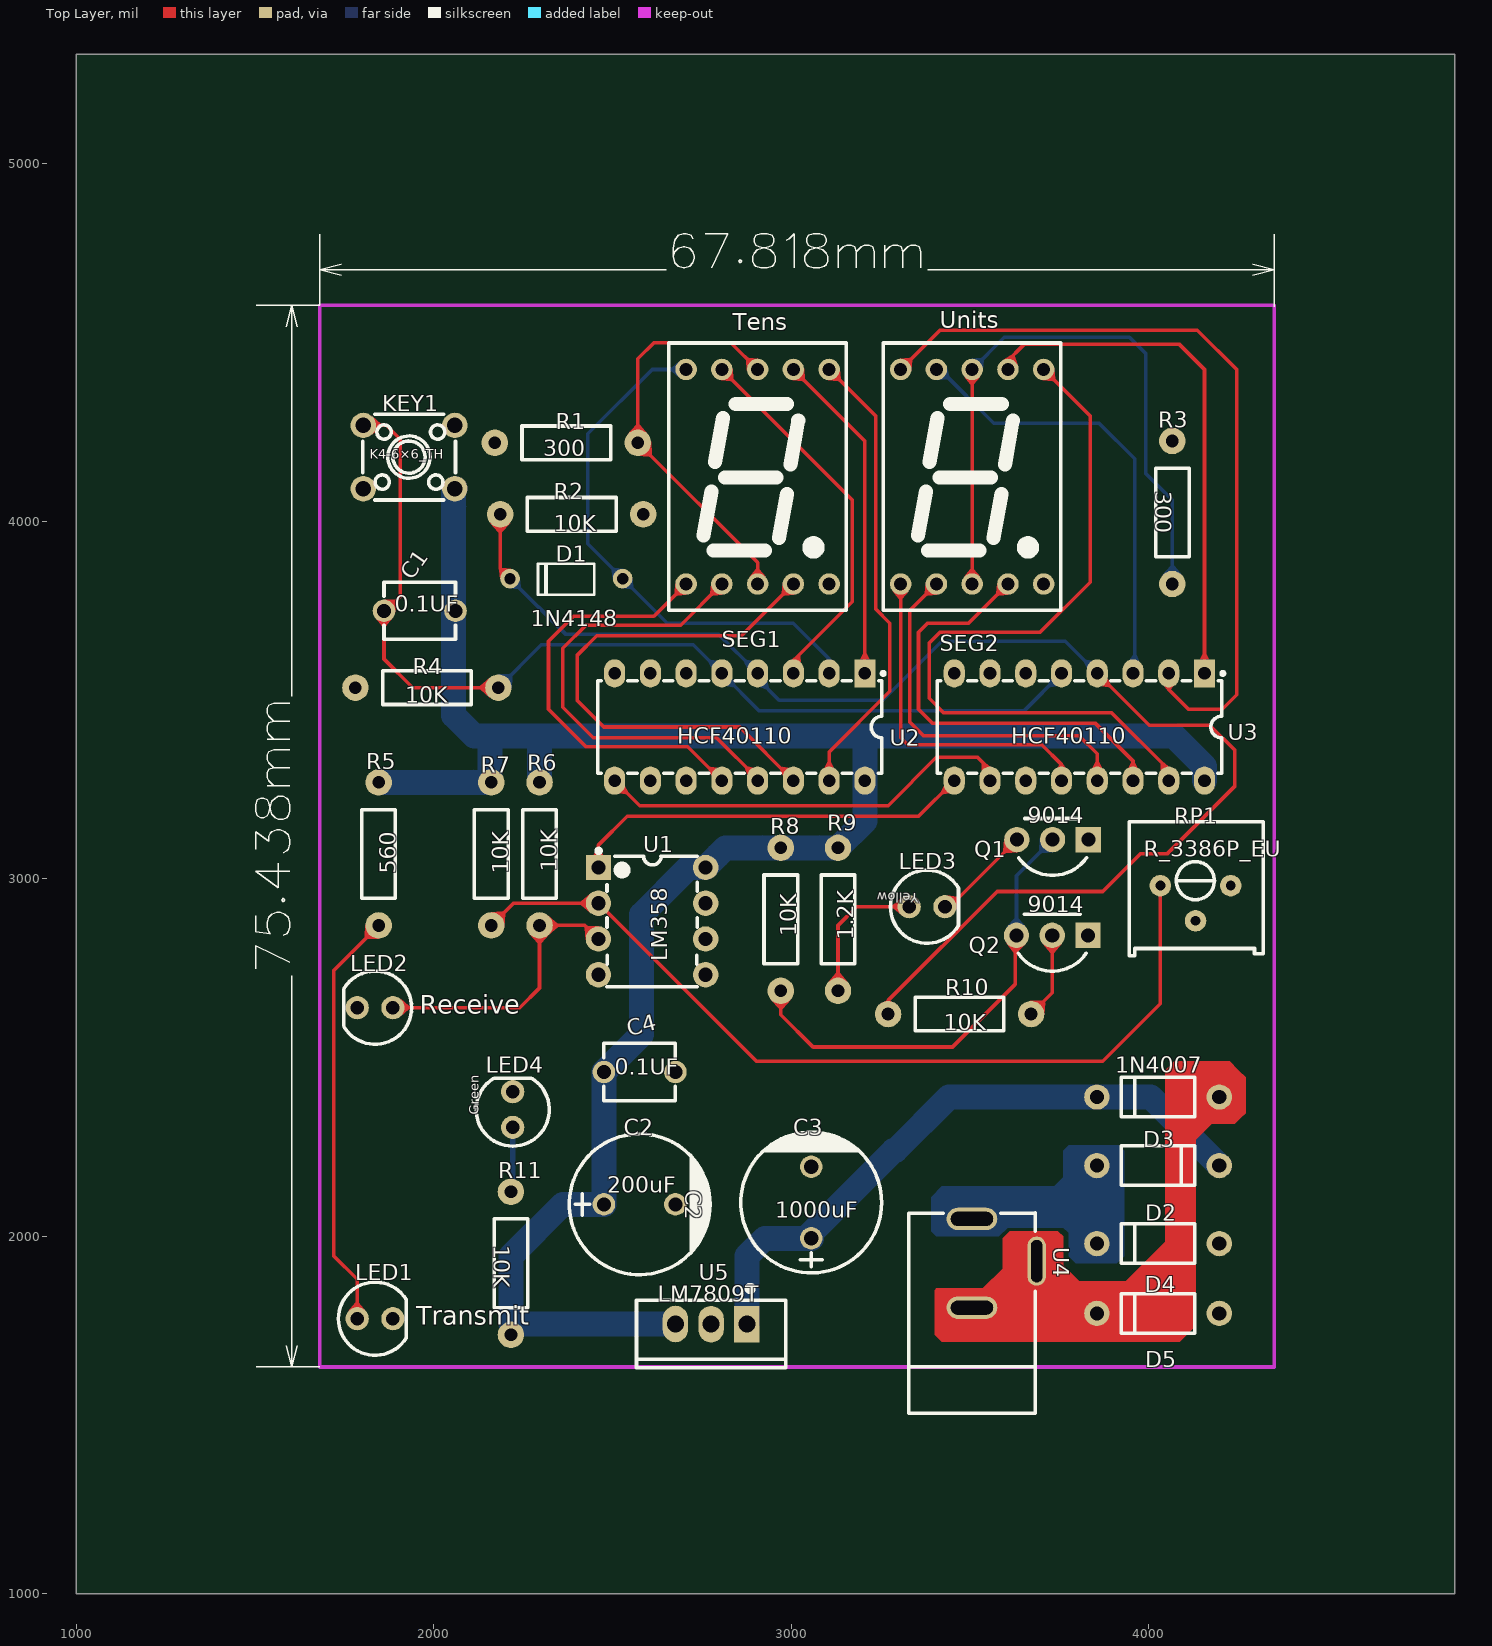
[diagram p0: Top Layer view]
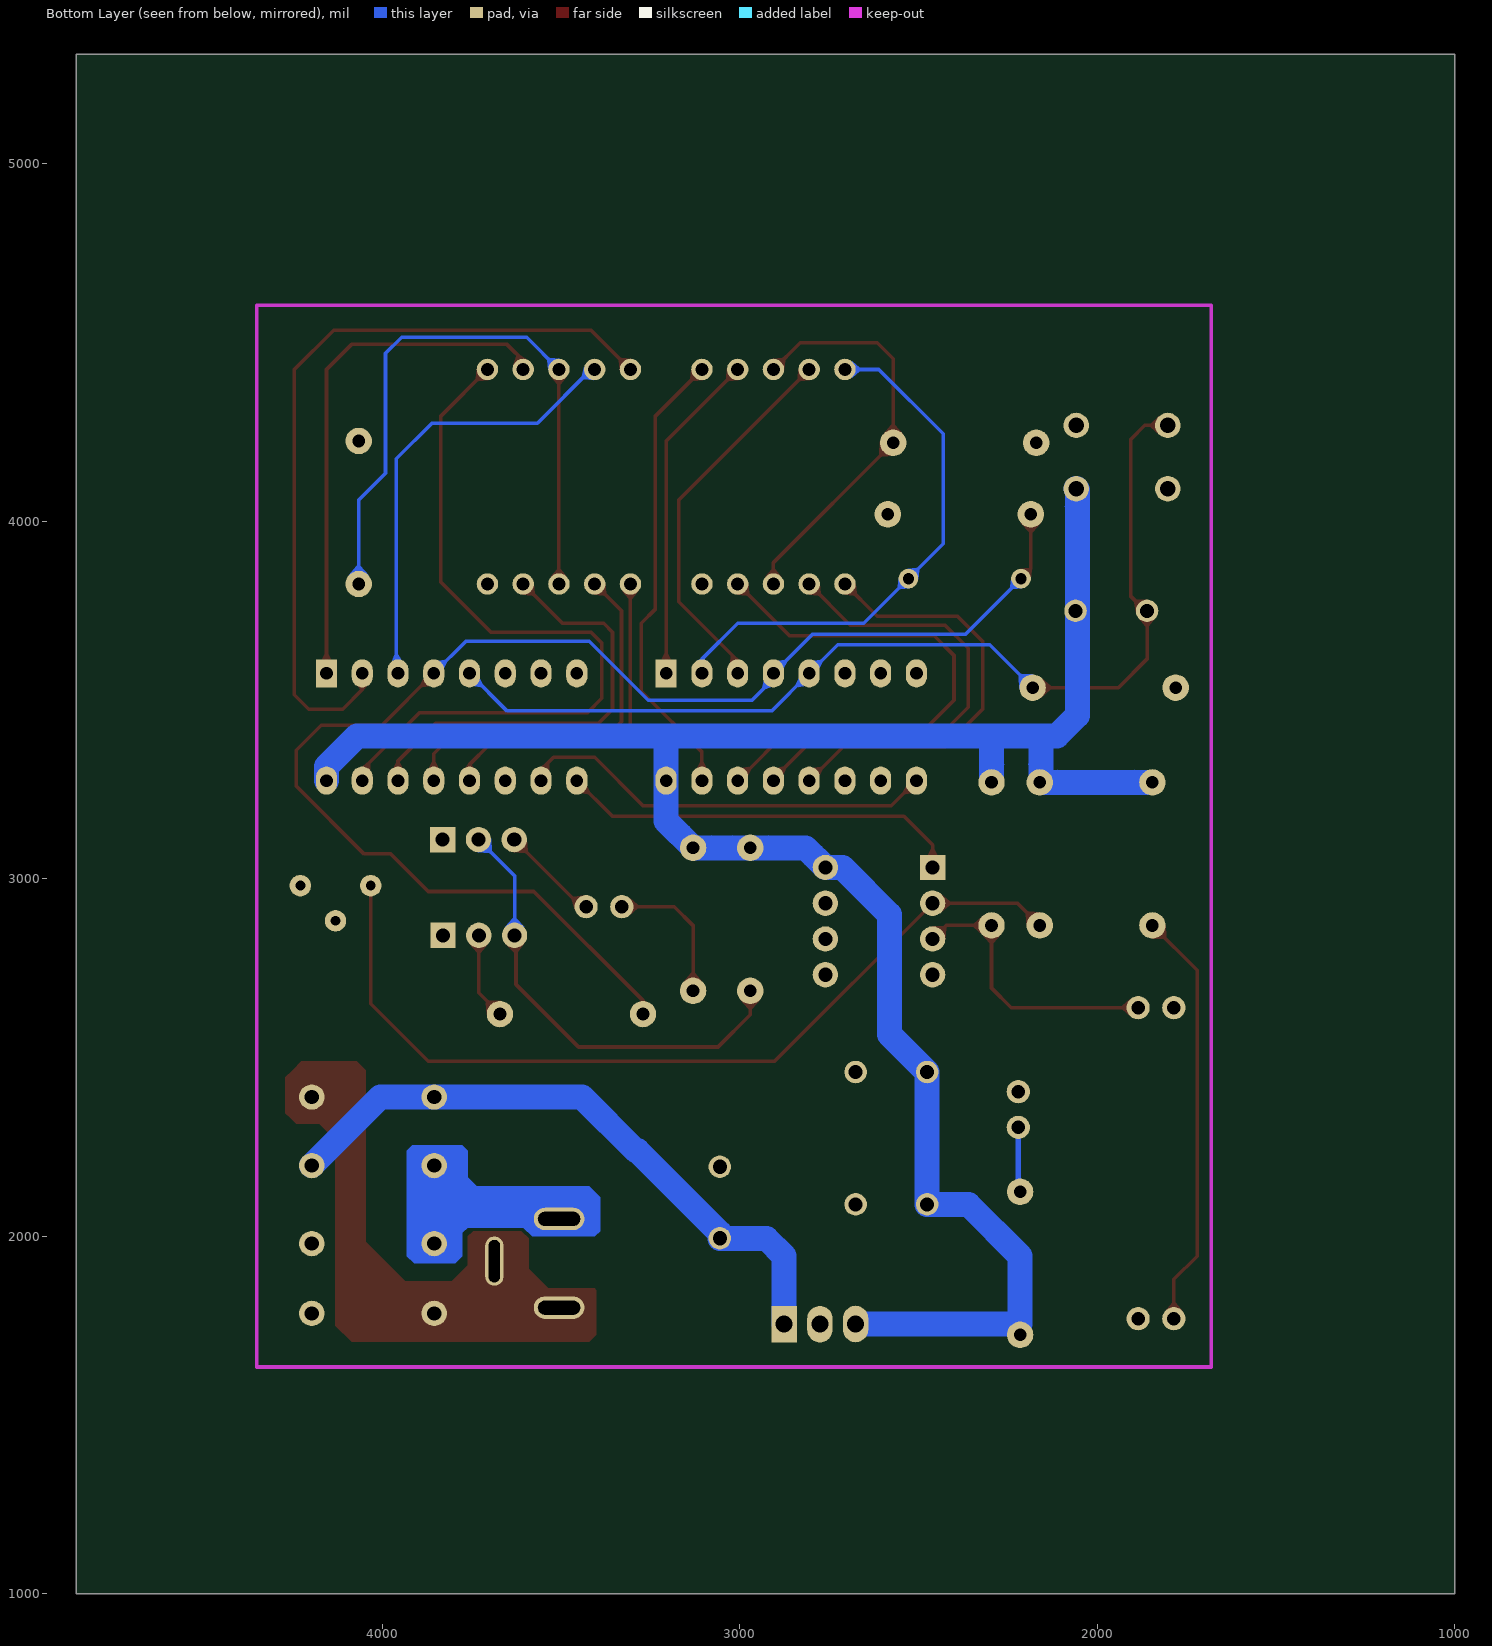
[diagram p1: Bottom Layer view, seen from below]
# Altium PCB MISC82671.pcbdoc
Units mil, origin at the board's own origin, x right, y up, seen from the top; angles counter-clockwise.
Board outline 3855.81 x 4306 mil, 2 copper layers (Top Layer, Bottom Layer); 37 components, 40 nets, 127 pads, 0 vias.

## Layer stack, top to bottom (the 12.6 mil dielectric is the usual default, probably not edited)
Top Solder: solder mask 0.4, Solder Resist, Dk 3.5
Top Layer: signal copper 1.4
Dielectric1: dielectric 12.6, FR-4, Dk 4.8
Bottom Layer: signal copper 1.4
Bottom Solder: solder mask 0.4, Solder Resist, Dk 3.5

## Board outline
4855.81,1000 1000,1000 1000,5306 4855.81,5306

## Design rules (kind name [scope] priority, off if disabled: settings)
Clearance [All] p1: gap=10
PolygonConnect [All] p1: connectstyle=Relief reliefconductorwidth=10 reliefentries=4 polygonreliefangle="90 Angle" airgapwidth=10
RoutingVias [All] p1: holewidth=28 width=50 viastyle="Through Hole" minholewidth=28 minwidth=50 maxholewidth=28 maxwidth=50
SolderMaskExpansion [All] p1: expansion=4
Width [All] p1: maxlimit=10 minlimit=10 preferedwidth=10
30 further rules are at their usual default settings.

## Components (designator, comment, footprint, x,y, rotation, side; value= is the part's Value field where it differs from the comment)
C1 "0.1UF" CAP-TH_L5.0-W4.0-P5.00-D1.0 1960.81,3749.3 r0 top
C2 "200uF" CAP-TH_BD10.0-P5.00-D1.0-FD 2575.81,2089.3 r0 top
C3 "1000uF" CAP-TH_BD10.0-P5.00-D1.0-FD 3055.81,2094.3 r90 top
C4 "0.1UF" CAP-TH_L5.0-W4.0-P5.00-D1.0 2575.81,2459.3 r180 top
D1 "1N4148" DO-35_BD2.2-L4.0-D0.50_1N4148 2370.81,3839.3 r180 top
D2 "1N4007" DO-41_BD2.4-L4.7-P8.70-D0.9-FD 4025.81,2197.52 r0 top
D3 "1N4007" DO-41_BD2.4-L4.7-P8.70-D0.9-FD 4025.81,2389.3 r180 top
D4 "1N4007" DO-41_BD2.4-L4.7-P8.70-D0.9-FD 4025.81,1979.3 r180 top
D5 "1N4007" DO-41_BD2.4-L4.7-P8.70-D0.9-FD 4025.81,1784.3 r180 top
KEY1 "K4-6×6_TH" KEY-TH_4P-L6.0-W6.0-P4.50-LS6.5 1930.81,4179.3 r180 top
LED1 "LED-TH-5mm_R" LED-TH_BD5.0_RED 1835.81,1769.3 r90 top
LED2 "LED-TH-5mm_R" LED-TH_BD5.0_RED 1835.81,2639.3 r270 top
LED3 "Yellow" LED-TH_BD5.0_RED 3379.83,2921.68 r90 top
LED4 "Green" LED-TH_BD5.0_RED 2220.81,2354.3 r180 top
Q1 "9014" TO-92-3_L4.9-W3.7-P2.54-L 3730.81,3109.3 r180 top
Q2 "9014" TO-92-3_L4.9-W3.7-P2.54-L 3729.83,2841.68 r180 top
R1 "300" R_AXIAL-0.4 2370.81,4219.3 r0 top
R2 "10K" R_AXIAL-0.4 2385.81,4019.3 r0 top
R3 "300" R_AXIAL-0.4 4065.81,4024.3 r270 top
R4 "10K" R_AXIAL-0.4 1980.81,3534.3 r0 top
R5 "560" R_AXIAL-0.4 1845.81,3069.3 r90 top
R6 "10K" R_AXIAL-0.4 2295.81,3069.3 r90 top
R7 "10K" R_AXIAL-0.4 2160.81,3069.3 r90 top
R8 "10K" R_AXIAL-0.4 2970.61,2886.38 r90 top
R9 "1.2K" R_AXIAL-0.4 3130.61,2886.38 r90 top
R10 "10K" R_AXIAL-0.4 3470.61,2621.38 r180 top
R11 "10K" R_AXIAL-0.4 2215.81,1924.3 r270 top
RP1 "R_3386P_EU" RES-ADJ-TH_3386P 4130.63,2931.41 r180 top
SEG1 "SEG-TH_0.56×1_Cathode" LED-SEG-TH_10P-L12.6-W19.0-P2.54-S15.24-BL 2905.81,4124.3 r0 top
SEG2 "SEG-TH_0.56×1_Cathode" LED-SEG-TH_10P-L12.6-W19.0-P2.54-S15.24-BL 3505.81,4124.3 r0 top
U1 "LM358" DIP-8_L8.8-W6.4-P2.54-LS7.6-BL 2610.61,2881.38 r270 top
U2 "HCF40110" DIP-16_16P-L20.2-W6.6-P2.54-LS7.6-BL 2855.81,3424.3 r180 top
U3 "HCF40110" DIP-16_16P-L20.2-W6.6-P2.54-LS7.6-BL 3805.81,3424.3 r180 top
U4 "HX DC005-2.5" DC-IN-TH_HX-DC005-2.5 3595.81,1924.3 r90 top
U5 "LM7809T" TO-220-3_L10.0-W4.5-P2.54-L 2775.81,1754.3 r180 top
? "" ? 1591.4,3119.3 r0 top
? "" ? 3015.81,4701.65 r0 top

## Footprints (in the part's own frame and the unit in brackets; to place one, negate y for a bottom-side part, rotate by r counter-clockwise, add the part's x,y. Pads: shape width x height; smd on the part's side, far side on the other; paste and mask are expansions set on the pad)
CAP-TH_BD10.0-P5.00-D1.0-FD [mm]
  round 1.6 hole 1 paste+0 mask+0.051: 1(-2.54,0) 2(2.54,0)
  silkscreen extent -5,-5 5.08,5
CAP-TH_L5.0-W4.0-P5.00-D1.0 [mm]
  round 1.6 hole 1 paste+0 mask+0.051: 1(-2.54,0) 2(2.54,0)
  silkscreen extent -2.54,-2.03 2.54,2.03
DC-IN-TH_HX-DC005-2.5 [mm]
  oval 3.5x1.3 hole 0.8 slot 3 at 0 deg paste+0 mask+0.05: 2(0.155,-2.3)
  oval 1.6x3.6 hole 1 slot 3 at 90 deg paste+0 mask+0.05: 3(-3.15,2.3) 4(3.15,2.3)
  silkscreen extent -10.65,-2.2 3.57,6.8
DIP-8_L8.8-W6.4-P2.54-LS7.6-BL [mm]
  rect 1.8x1.8 hole 1 paste+0 mask+0.051: 1(-3.81,-3.81)
  round 1.8 hole 1 paste+0 mask+0.051: 2(-1.27,-3.81) 3(1.27,-3.81) 4(3.81,-3.81) 5(3.81,3.81) 6(1.27,3.81) 7(-1.27,3.81) 8(-3.81,3.81)
  silkscreen extent -5.14,-3.95 4.66,3.2
DIP-16_16P-L20.2-W6.6-P2.54-LS7.6-BL [mm]
  rect 1.5x2 hole 0.9 paste+0 mask+0.051: 1(-8.89,-3.81)
  oval 1.5x2 hole 0.9 paste+0 mask+0.051: 2(-6.35,-3.81) 3(-3.81,-3.81) 4(-1.27,-3.81) 5(1.27,-3.81) 6(3.81,-3.81) 7(6.35,-3.81) 8(8.89,-3.81) 9(8.89,3.81) 10(6.35,3.81) 11(3.81,3.81) 12(1.27,3.81) 13(-1.27,3.81) 14(-3.81,3.81) 15(-6.35,3.81) 16(-8.89,3.81)
  silkscreen extent -10.31,-3.93 10.1,3.3
DO-35_BD2.2-L4.0-D0.50_1N4148 [mm]
  round 1.4 hole 0.8 paste+0 mask+0.05: 1(-4,0) 2(4,0)
  silkscreen extent -1.98,-1.06 2.02,1.14
DO-41_BD2.4-L4.7-P8.70-D0.9-FD [mm]
  round 1.8 hole 1 paste+0 mask+0.051: 1(-4.35,0) 2(4.35,0)
  silkscreen extent -2.6,-1.4 2.6,1.4
KEY-TH_4P-L6.0-W6.0-P4.50-LS6.5 [mm]
  round 1.8 hole 1.1 paste+0 mask+0.051: 1(-3.251,-2.25) 2(3.251,-2.25) 3(3.251,2.25) 4(-3.251,2.25)
  silkscreen extent -3.3,-3.05 3.3,3.05
LED-SEG-TH_10P-L12.6-W19.0-P2.54-S15.24-BL [mil]
  round 60 hole 36 paste+0 mask+2: 1(-200,-300) 2(-100,-300) 3(0,-300) 4(100,-300) 5(200,-300) 6(200,300) 7(100,300) 8(0,300) 9(-100,300) 10(-200,300)
  silkscreen extent -248,-374 248,374
LED-TH_BD5.0_RED [mil]
  round 65 hole 38 paste+0 mask+2: 1(0,50) 2(0,-50)
  silkscreen extent -102,-88 102,102
R_AXIAL-0.4 [mil]
  round 74 hole 35.4 paste+0 mask+2: 1(-200,0) 2(200,0)
  silkscreen extent -124,-47 124,47
RES-ADJ-TH_3386P [mil]
  round 60 hole 27.56 paste+0 mask+2: 1(98.43,-49.21) 2(0.01,49.22) 3(-98.42,-49.21)
  silkscreen extent -190,-228 185,147
TO-92-3_L4.9-W3.7-P2.54-L [mm]
  rect 1.8x1.8 hole 1 paste+0 mask+0.051: 1(-2.54,0)
  round 1.8 hole 1 paste+0 mask+0.051: 2(0,0) 3(2.54,0)
  silkscreen extent -2.41,-1.5 2.41,2.54
TO-220-3_L10.0-W4.5-P2.54-L [mm]
  rect 1.8x2.6 hole 1.2 paste+0 mask+0.051: 1(-2.54,0.005)
  oval 1.8x2.6 hole 1.2 paste+0 mask+0.051: 2(0,0.005) 3(2.54,-0.005)
  silkscreen extent -5.3,-2.73 5.3,3.09
? [mil]
  silkscreen extent -89,-1485 89,1485

## Nets (pads, with @x,y where several pads share a name; then routed paths per layer and width w, separated by ;. In a path a pad name is that pad's centre, name@x,y a point inside that pad or via, vN(x,y) a via of type N, cw(c..) or ccw(c..) an arc to the next point about the centre after c; other vN are vias at no path point)
+9V: C1.2 C2.1 C4.2 KEY1.4 R5.2 R6.2 R7.2 R8.2 R9.2 R11.2 U1.8 U2.16 U3.16 U5.3 | length 6205.2
  Bottom Layer w70: R5.2 R7.2 2157.67,3272.44 2157.67,3399.3 ; KEY1.4 2055.81,4087.7 2055.81,3456.7 2113.21,3399.3 4070.81,3399.3 4155.81,3314.3 U3.16 ; R6.2 2295.81,3399.3 ; U5.3 2215.81,1754.49 2215.81,1944.3 2360.81,2089.3 C2.1 C4.2 2580.81,2564.3 2580.81,2899.3 2712.91,3031.4 U1.8 2815.61,3086.4 R8.2 R9.2 3205.81,3161.6 U2.16 3205.61,3399.3
D3_2: C3.1 D2.2 D3.2 U5.1 | length 1784.1
  Bottom Layer w70: U5.1 2875.82,1944.31 2925.81,1994.3 C3.1 3055.81,2009.3 3285.81,2239.3 3290.81,2239.3 3440.81,2389.3 D3.2 4005.31,2389.3 D2.2
GND: C2.2 C3.2 C4.1 D4.1 D5.1 LED1.2 LED2.2 LED4.2 Q1.1 Q2.1 R1.1 R2.2 R3.1 R4.1 RP1.2 RP1.3 U1.4 U2.6 U2.7 U2.8 U3.6 U3.7 U3.8 U5.2
LED1_1: LED1.1 R5.1 | length 1178.7
  Top Layer w10: LED1.1 1785.81,1879.3 1720.81,1944.3 1720.81,2744.3 R5.1
LED3_2: LED3.2 Q1.3 | length 278.7
  Top Layer w10: LED3.2 3443.19,2921.68 Q1.3
Q2_2: Q2.2 R10.1 | length 244.8
  Top Layer w10: R10.1 3729.83,2680.6 Q2.2
R3_2: R3.2 SEG2.3 SEG2.8 | length 1817
  Top Layer w10: SEG2.3 SEG2.8
  Bottom Layer w10: SEG2.8 3595.81,4514.3 3945.81,4514.3 3990.81,4469.3 3990.81,4134.3 4065.81,4059.3 R3.2
R8_1: Q1.2 Q2.3 R8.1 | length 1280.5
  Top Layer w10: R8.1 2970.61,2619.5 3060.81,2529.3 3450.81,2529.3 3625.81,2704.3 3625.81,2837.7 Q2.3
  Bottom Layer w10: Q2.3 3629.83,3008.32 Q1.2
R9_1: LED3.1 R9.1 | length 403.7
  Top Layer w10: R9.1 3130.61,2869.1 3183.21,2921.7 LED3.1
R11_1: LED4.1 R11.1 | length 182.1
  Bottom Layer w15: R11.1 2220.81,2129.3 LED4.1
S$4459: 
S$4463: 
SEG1_3: R1.2 SEG1.3 SEG1.8 | length 1153.5
  Top Layer w10: SEG1.3 2905.81,3884.3 R1.2 2570.81,4454.3 2615.81,4499.3 2830.81,4499.3 SEG1.8
SEG1_5: SEG1.5
SEG2_1: SEG2.1 U3.12 | length 956.1
  Top Layer w10: SEG2.1 3305.81,3394.3 3325.81,3374.3 3700.81,3374.3 3755.81,3319.3 U3.12
SEG2_2: SEG2.2 U3.13 | length 1053.3
  Top Layer w10: SEG2.2 3330.81,3749.3 3330.81,3439.3 3370.81,3399.3 3805.81,3399.3 3855.81,3349.3 U3.13
SEG2_4: SEG2.4 U3.14 | length 1236
  Top Layer w10: SEG2.4 3495.81,3714.3 3380.81,3714.3 3355.81,3689.3 3355.81,3474.3 3395.81,3434.3 3850.81,3434.3 3955.81,3329.3 U3.14
SEG2_5: SEG2.5
SEG2_6: SEG2.6 U3.15 | length 2107.1
  Top Layer w10: SEG2.6 3835.81,4294.3 3835.81,3829.3 3695.81,3689.3 3415.81,3689.3 3385.81,3659.3 3385.81,3504.3 3425.81,3464.3 3895.81,3464.3 4055.81,3304.3 U3.15
SEG2_7: SEG2.7 U3.1 | length 1476.8
  Top Layer w10: SEG2.7 3600.81,4429.3 3600.81,4444.3 3650.81,4494.3 4085.81,4494.3 4155.81,4424.3 U3.1
SEG2_9: SEG2.9 U3.3 | length 1260.6
  Bottom Layer w10: SEG2.9 3415.81,4424.3 3565.81,4274.3 3860.81,4274.3 3960.81,4174.3 3960.81,3579.3 U3.3
SEG2_10: SEG2.10 U3.2 | length 2215.5
  Top Layer w10: SEG2.10 3415.81,4534.3 4135.81,4534.3 4245.81,4424.3 4245.81,3514.3 4205.81,3474.3 4110.81,3474.3 4055.81,3529.3 U3.2
U1_1: U1.1 U3.9 | length 1132.5
  Top Layer w10: U1.1 2460.61,3094.1 2540.81,3174.3 3355.81,3174.3 U3.9
U1_2: R7.1 RP1.1 U1.2 | length 2477
  Top Layer w10: R7.1 2222.89,2931.38 U1.2 2902.69,2489.3 3870.81,2489.3 4032.18,2650.68 RP1.1
U1_3: LED2.1 R6.1 U1.3 | length 788.3
  Top Layer w10: LED2.1 2240.81,2639.3 2295.81,2694.3 R6.1 2422.71,2869.3 U1.3
U2_1: SEG1.7 U2.1 | length 932.8
  Top Layer w10: SEG1.7 3205.81,4224.3 U2.1
U2_2: D1.1 SEG1.10 U2.2 | length 1505.6
  Bottom Layer w10: SEG1.10 2610.81,4424.3 2430.81,4244.3 2430.81,3936.78 D1.1 2653.31,3714.3 3005.81,3714.3 3105.81,3614.3 U2.2
U2_3: SEG1.9 U2.3 | length 1069.5
  Top Layer w10: SEG1.9 3170.81,4059.3 3170.81,3774.3 3005.81,3609.3 U2.3
U2_4: D1.2 R2.1 R10.2 U2.4 U3.4 | length 3919.7
  Top Layer w10: R2.1 2185.81,3866.82 D1.2 ; R10.2 3270.61,2659.1 3575.81,2964.3 3870.81,2964.3 3975.81,3069.3 4050.81,3069.3 4240.81,3259.3 4240.81,3359.3 4170.81,3429.3 4000.81,3429.3 U3.4
  Bottom Layer w10: D1.2 2368.31,3684.3 2795.81,3684.3 U2.4 2905.81,3559.3 2965.81,3499.3 3255.81,3499.3 3420.81,3664.3 3765.81,3664.3 U3.4
U2_5: C1.1 KEY1.2 R4.2 U2.5 U3.5 | length 2853.5
  Top Layer w10: KEY1.2 1867.21,4267.9 1905.81,4229.3 1905.81,3789.3 1865.81,3749.3 C1.1 1860.81,3614.3 1940.81,3534.3 R4.2
  Bottom Layer w10: R4.2 2300.81,3654.3 2725.81,3654.3 U2.5 2910.81,3469.3 3650.81,3469.3 U3.5
U2_9: U2.9 U3.10 | length 1179.4
  Top Layer w10: U2.9 2575.81,3204.3 3270.81,3204.3 3405.81,3339.3 3520.81,3339.3 3555.81,3304.3 U3.10
U2_10: U2.10
U2_11: U2.11
U2_12: SEG1.1 U2.12 | length 1209.1
  Top Layer w10: SEG1.1 2615.81,3734.3 2390.81,3734.3 2320.81,3664.3 2320.81,3474.3 2425.81,3369.3 2710.81,3369.3 U2.12
U2_13: SEG1.2 U2.13 | length 1317.4
  Top Layer w10: SEG1.2 2690.81,3709.3 2425.81,3709.3 2360.81,3644.3 2360.81,3479.3 2445.81,3394.3 2790.81,3394.3 2905.81,3279.3 U2.13
U2_14: SEG1.4 U2.14 | length 1511
  Top Layer w10: U2.14 2855.81,3424.3 2475.81,3424.3 2400.81,3499.3 2400.81,3624.3 2455.81,3679.3 2860.81,3679.3 SEG1.4
U2_15: SEG1.6 U2.15 | length 1290.8
  Top Layer w10: U2.15 3105.81,3354.3 3275.81,3524.3 3275.81,3714.3 3235.81,3754.3 3235.81,4294.3 SEG1.6
U3_11: U3.11
U4_3: D3.1 D5.2 U4.2 U4.3
U4_4: D2.1 D4.2 U4.4
pads on no net: KEY1.1 KEY1.3 U1.5 U1.6 U1.7

## Other copper
Top Layer:
  region net SEG2_10: 4068.31,3537.71 4043.31,3537.71 4050.81,3529.3 4060.81,3529.3
  region net U2_4: 3884.85,3559.15 3870.37,3538.77 3886.9,3536.14 3892.78,3544.4
  region net SEG2_6: 4055.81,3313.67 4033.16,3303.09 4033.32,3319.72 4042.95,3324.22
  region net SEG2_4: 3968.31,3310.89 3943.31,3310.89 3950.81,3325.89 3960.81,3325.89
  region net SEG2_2: 3868.31,3310.89 3843.31,3310.89 3850.81,3325.89 3860.81,3325.89
  region net SEG2_1: 3768.31,3310.89 3743.31,3310.89 3750.81,3319.3 3760.81,3319.3
  region net U2_9: 3555.81,3313.67 3533.16,3303.09 3533.32,3319.72 3542.95,3324.22
  region net U1_1: 3441.24,3238.77 3426.76,3259.15 3418.84,3244.4 3424.71,3236.14
  region net U2_3: 3026.62,3605.09 3003.1,3613.55 3014.74,3625.3 3025.14,3621.56
  region net U2_15: 3118.31,3310.89 3093.31,3310.89 3100.81,3325.89 3110.81,3325.89
  region net U2_14: 2991.24,3309.83 2976.76,3289.45 2968.84,3304.2 2974.71,3312.46
  region net U2_13: 2893.49,3310.98 2877.32,3291.91 2870.72,3307.32 2877.21,3314.97
  region net U2_12: 2791.24,3309.83 2776.76,3289.45 2768.84,3304.2 2774.71,3312.46
  region net U2_9: 2534.85,3259.15 2520.37,3238.77 2536.9,3236.14 2542.78,3244.4
  region net SEG2_7: 4143.31,3613.67 4168.31,3613.67 4160.81,3628.67 4150.81,3628.67
  region net U2_1: 3193.31,3613.67 3218.31,3613.67 3210.81,3628.67 3200.81,3628.67
  region net U1_1: 2448.11,3066.81 2473.11,3066.81 2465.61,3081.81 2455.61,3081.81
  region net U1_3: 2425.24,2829.17 2462.83,2866.74 2430.04,2869.04 2422.97,2861.97
  region net U1_2: 2437.17,2957.96 2437.17,2904.81 2412.37,2926.38 2412.37,2936.38
  region net SEG2_10: 3303.93,4454.24 3335.75,4422.42 3338.22,4449.64 3331.15,4456.72
  region net R3_2: 3528.31,4404.46 3483.31,4404.46 3500.81,4383.46 3510.81,4383.46
  region net SEG2_7: 3633.61,4435.57 3591.15,4450.48 3614.11,4464.67 3624.57,4461
  region net SEG2_6: 3703.93,4394.36 3735.75,4426.18 3738.22,4398.96 3731.15,4391.88
  region net SEG2_4: 3575.86,3826.18 3607.68,3794.36 3580.46,3791.88 3573.39,3798.96
  region net R3_2: 3528.31,3844.14 3483.31,3844.14 3500.81,3865.14 3510.81,3865.14
  region net SEG2_2: 3375.86,3826.18 3407.68,3794.36 3380.46,3791.88 3373.39,3798.96
  region net SEG2_1: 3328.31,3804.46 3283.31,3804.46 3300.81,3783.46 3310.81,3783.46
  region net U2_3: 2803.93,4394.36 2835.75,4426.18 2838.22,4398.96 2831.15,4391.88
  region net SEG1_3: 2875.86,4422.42 2907.68,4454.24 2880.46,4456.72 2873.39,4449.64
  region net U2_1: 3003.93,4394.36 3035.75,4426.18 3038.22,4398.96 3031.15,4391.88
  region net U2_15: 3103.93,4394.36 3135.75,4426.18 3138.22,4398.96 3131.15,4391.88
  region net U2_14: 2975.86,3826.18 3007.68,3794.36 2980.46,3791.88 2973.39,3798.96
  region net SEG1_3: 2928.31,3844.14 2883.31,3844.14 2900.81,3865.14 2910.81,3865.14
  region net U2_13: 2775.86,3826.18 2807.68,3794.36 2780.46,3791.88 2773.39,3798.96
  region net U2_12: 2675.86,3826.18 2707.68,3794.36 2680.46,3791.88 2673.39,3798.96
  region net U2_4: 3298.36,2645.85 3242.86,2645.85 3265.61,2659.1 3275.61,2659.1
  region net Q2_2: 3668.29,2658.31 3707.53,2619.06 3709.76,2653.46 3702.69,2660.53
  region net R9_1: 3158.36,2710.85 3102.86,2710.85 3125.61,2736.75 3135.61,2736.75
  region net R8_1: 2998.36,2661.91 2942.86,2661.91 2965.61,2636.01 2975.61,2636.01
  region net U1_2: 2158.49,2906.23 2197.73,2866.98 2199.96,2901.38 2192.89,2908.45
  region net U1_3: 2323.56,2844.83 2268.06,2844.83 2290.81,2818.93 2300.81,2818.93
  region net U1_3: 2320.28,2841.55 2320.28,2897.05 2346.18,2874.3 2346.18,2864.3
  region net LED1_1: 1808.88,2871.62 1848.12,2832.37 1813.72,2830.15 1806.65,2837.22
  region net U2_5: 2156.33,3506.55 2156.33,3562.05 2130.43,3539.3 2130.43,3529.3
  region net U2_4: 2213.56,3994.83 2158.06,3994.83 2180.81,3968.93 2190.81,3968.93
  region net SEG1_3: 2598.56,4243.77 2543.06,4243.77 2565.81,4269.67 2575.81,4269.67
  region net SEG1_3: 2568.49,4182.37 2607.73,4221.62 2609.96,4187.22 2602.89,4180.15
  region net R8_1: 3654.35,2816.11 3601.39,2820.54 3620.81,2794.03 3630.81,2793.19
  region net Q2_2: 3756.4,2818.25 3703.25,2818.24 3724.83,2793.44 3734.83,2793.44
  region net LED3_2: 3595.44,3111.52 3633.02,3073.94 3600.23,3071.65 3593.16,3078.73
  region net LED3_2: 3461.08,2912.77 3434.76,2953.8 3464.31,2949.87 3469.83,2941.26
  region net R9_1: 3308.34,2946.06 3308.32,2897.31 3285.58,2916.7 3285.58,2926.7
  region net U1_3: 1907.3,2614.93 1907.3,2663.68 1930.05,2644.3 1930.05,2634.3
  region net LED1_1: 1810.18,1790.8 1761.43,1790.8 1780.81,1813.55 1790.81,1813.55
  region net U2_5: 1826.24,4241.33 1826.24,4294.48 1851.05,4272.9 1851.05,4262.9
  region net U2_4: 2185.82,3837.57 2215.05,3866.8 2190.33,3869.37 2183.26,3862.3
  region net U2_5: 1884.43,3728.47 1837.18,3728.47 1855.81,3706.42 1865.81,3706.42
  region net U2_5: 1891.97,3744.74 1861.43,3780.79 1890.28,3780.85 1896.77,3773.19
  region net U4_3: 3405.81,1854.3 3535.81,1854.3 3590.81,1909.3 3590.81,1994.3 3610.81,2014.3 3730.81,2014.3 3745.81,2014.3 3760.81,1999.3 3760.81,1919.3 3805.81,1874.3 3905.81,1874.3 3935.81,1874.3 3995.81,1934.3 4045.81,1984.3 4045.81,2464.3 4070.81,2489.3 4225.81,2489.3 4250.81,2464.3 4270.81,2444.3 4270.81,2344.3 4255.81,2329.3 4240.81,2314.3 4175.81,2314.3 4130.81,2269.3 4130.81,1749.3 4085.81,1704.3 3420.81,1704.3 3400.81,1724.3 3400.81,1849.3 3405.81,1854.3
Bottom Layer:
  region net SEG2_9: 3971.42,3609.21 3946.6,3612.2 3955.81,3626.2 3965.81,3624.99
  region net U2_4: 3841.24,3609.83 3826.76,3589.45 3818.84,3604.2 3824.71,3612.46
  region net U2_5: 3741.24,3538.77 3726.76,3559.15 3718.84,3544.4 3724.71,3536.14
  region net U2_2: 3118.31,3610.89 3093.31,3610.89 3100.81,3614.3 3110.81,3614.3
  region net U2_4: 2891.24,3609.83 2876.76,3589.45 2868.84,3604.2 2874.71,3612.46
  region net U2_4: 2932.57,3551.99 2913.42,3535.93 2928.79,3529.24 2936.48,3535.69
  region net U2_5: 2791.24,3609.83 2776.76,3589.45 2768.84,3604.2 2774.71,3612.46
  region net U2_5: 2834.85,3559.15 2820.37,3538.77 2836.9,3536.14 2842.78,3544.4
  region net +9V: 2758.38,3066.74 2795.97,3029.17 2819.46,3040.76 2769.95,3090.24
  region net SEG2_9: 3434.97,4431.33 3409.14,4394.49 3436.34,4396.7 3442.16,4405.01
  region net R3_2: 3503.93,4454.24 3535.75,4422.42 3538.22,4449.64 3531.15,4456.72
  region net U2_2: 2685.96,4401.8 2685.96,4446.8 2664.96,4429.3 2664.96,4419.3
  region net +9V: 3128.28,3123.31 3167.53,3084.07 3190.97,3097.27 3141.46,3146.75
  region net +9V: 3106.13,3058.63 3106.13,3114.13 3080.23,3121.38 3080.23,3051.38
  region net +9V: 2946.14,3114.14 2946.12,3058.64 2920.22,3051.4 2920.25,3121.4
  region net +9V: 2995.08,3058.63 2995.08,3114.13 3020.98,3121.38 3020.98,3051.38
  region net +9V: 2136.33,3241.55 2136.33,3297.05 2110.43,3304.3 2110.43,3234.3
  region net +9V: 2186.98,3295.45 2131.59,3292 2122.67,3317.39 2192.67,3321.76
  region net +9V: 2323.56,3293.77 2268.06,3293.77 2260.81,3319.67 2330.81,3319.67
  region net +9V: 1870.28,3241.55 1870.28,3297.05 1896.18,3304.3 1896.18,3234.3
  region net U2_5: 2178.49,3571.23 2217.73,3531.98 2219.96,3566.38 2212.89,3573.45
  region net R3_2: 4093.56,3848.77 4038.06,3848.77 4060.81,3874.67 4070.81,3874.67
  region net R8_1: 3656.4,2865.11 3603.25,2865.12 3624.83,2889.92 3634.83,2889.92
  region net R8_1: 3695.44,3111.52 3733.02,3073.94 3700.23,3071.65 3693.16,3078.72
  region net +9V: 2083.87,4065.65 2030.83,4068.96 2020.81,4044.73 2090.81,4040.37
  region net U2_2: 2500.78,3837.57 2530.01,3866.8 2505.29,3869.37 2498.22,3862.3
  region net U2_2: 2526.57,3811.79 2555.79,3841.04 2558.36,3816.32 2551.29,3809.24
  region net U2_4: 2211.59,3811.8 2240.83,3841.02 2243.38,3816.29 2236.31,3809.23
  region net U4_4: 3390.81,2109.3 3420.81,2139.3 3715.81,2139.3 3735.81,2139.3 3760.81,2164.3 3760.81,2239.3 3775.81,2254.3 3915.81,2254.3 3925.81,2244.3 3930.81,2239.3 3930.81,1944.3 3910.81,1924.3 3800.81,1924.3 3795.81,1924.3 3775.81,1944.3 3775.81,2009.3 3760.81,2024.3 3605.81,2024.3 3580.81,1999.3 3405.81,1999.3 3390.81,2014.3

## Silkscreen, mask and mechanical layers (free items; w line width, h text height)
Top Overlay:
  text "Units" at 3415.81,4524.3 h80
  text "Tens" at 2835.81,4519.3 h80
  text "Receive" at 1960.81,2604.3 h90
  text "C2" at 2530.81,2281.8 h45
  text "Transmit" at 1950.81,1734.3 h90